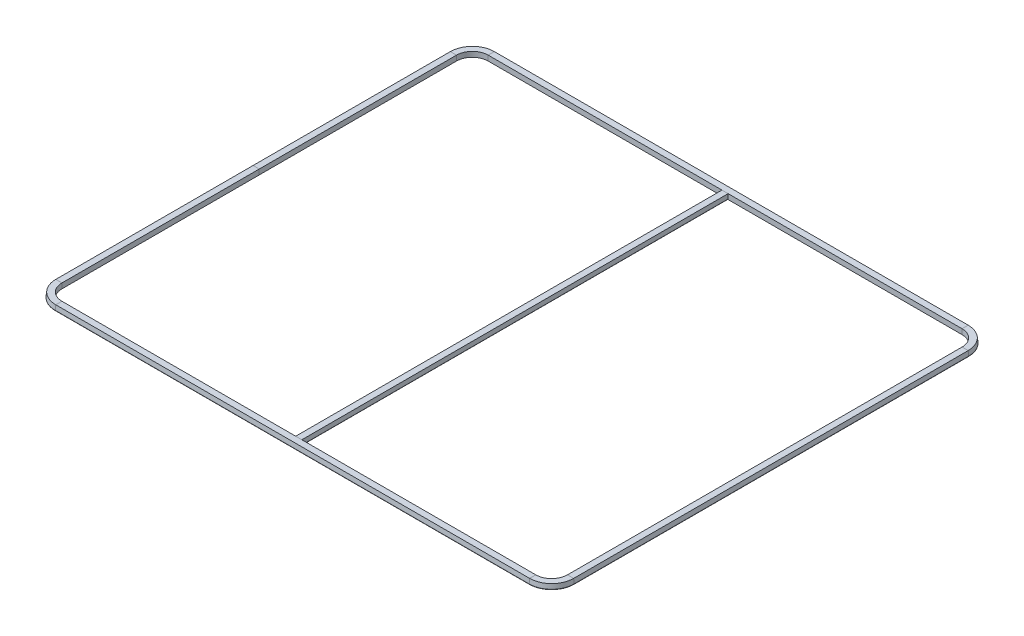
SolidWorks part; units mm, degrees
material "橡胶"
ref_plane "前视基准面" through (0, 0, 0) normal (0, 0, 1) x (1, 0, 0)
ref_plane "上视基准面" through (0, 0, 0) normal (0, 1, 0) x (1, 0, 0)
ref_plane "右视基准面" through (0, 0, 0) normal (1, 0, 0) x (0, 0, -1)
sketch "草图1" plane through (0, 0, 0) normal (0, 1, 0) x (1, 0, 0)
  line L1 (-1195, -1090) -> (1195, -1090)
  line L2 (-1290, -995) -> (-1290, 995)
  line L3 (-1195, 1090) -> (1195, 1090)
  line L4 (1290, -995) -> (1290, 995)
  line L5 (-1290, -1090) -> (1290, 1090) construction
  line L6 (-1290, 1090) -> (1290, -1090) construction
  arc A0 (1195, -1090) -> (1290, -995) centre (1195, -995) ccw
  arc A1 (-1290, 995) -> (-1195, 1090) centre (-1195, 995) cw
  arc A2 (-1195, -1090) -> (-1290, -995) centre (-1195, -995) cw
  arc A3 (1195, 1090) -> (1290, 995) centre (1195, 995) cw
  point P0 (0, 0)
  dimension "D3" = 95
  dimension "D1" = 2180
  dimension "D2" = 2580
sketch "草图2" plane through (0, 0, 0) normal (0, 0, 1) x (1, 0, 0)
  line L0 (-1275, 0) -> (-1305.6339, 0)
  line L1 (-1195, 0) -> (1195, 0) construction
  line L2 (-1308.6142, 3.3439) -> (-1306, 26)
  line L3 (-1306, 26) -> (-1275, 26)
  line L4 (-1275, 26) -> (-1275, 0)
  line L5 (-1290, 0) -> (-1290, 26) construction
  line L6 (-1290, 0) -> (1290, 0) construction
  arc A0 (-1305.6339, 0) -> (-1308.6142, 3.3439) centre (-1305.6339, 3) cw
  point P17 (-1309, 0)
  dimension "D5" = 3
  dimension "D1" = 26
  dimension "D2" = 3
  dimension "D3" = 31
  dimension "D4" = 15
sweep "扫描1" add profiles "草图2" path "草图1"
sketch "草图3" plane through (0, 0, 0) normal (0, 0, 1) x (1, 0, 0)
  line L0 (-16, 26) -> (-19, 0)
  line L1 (1195, 26) -> (-1195, 26) construction
  line L2 (1195, 0) -> (-1195, 0) construction
  line L3 (-19, 0) -> (15, 0)
  line L4 (15, 0) -> (15, 26)
  line L5 (15, 26) -> (-16, 26)
  line L6 (0, 26) -> (0, 0) construction
  dimension "D1" = 15
  dimension "D2" = 31
  dimension "D3" = 34
extrude "凸台-拉伸1" add sketch "草图3" along normal up to next and the other way up to next separate body
fillet "圆角1" radius 3 2 edges at (15, 0, 0) (-19, 0, 0)
